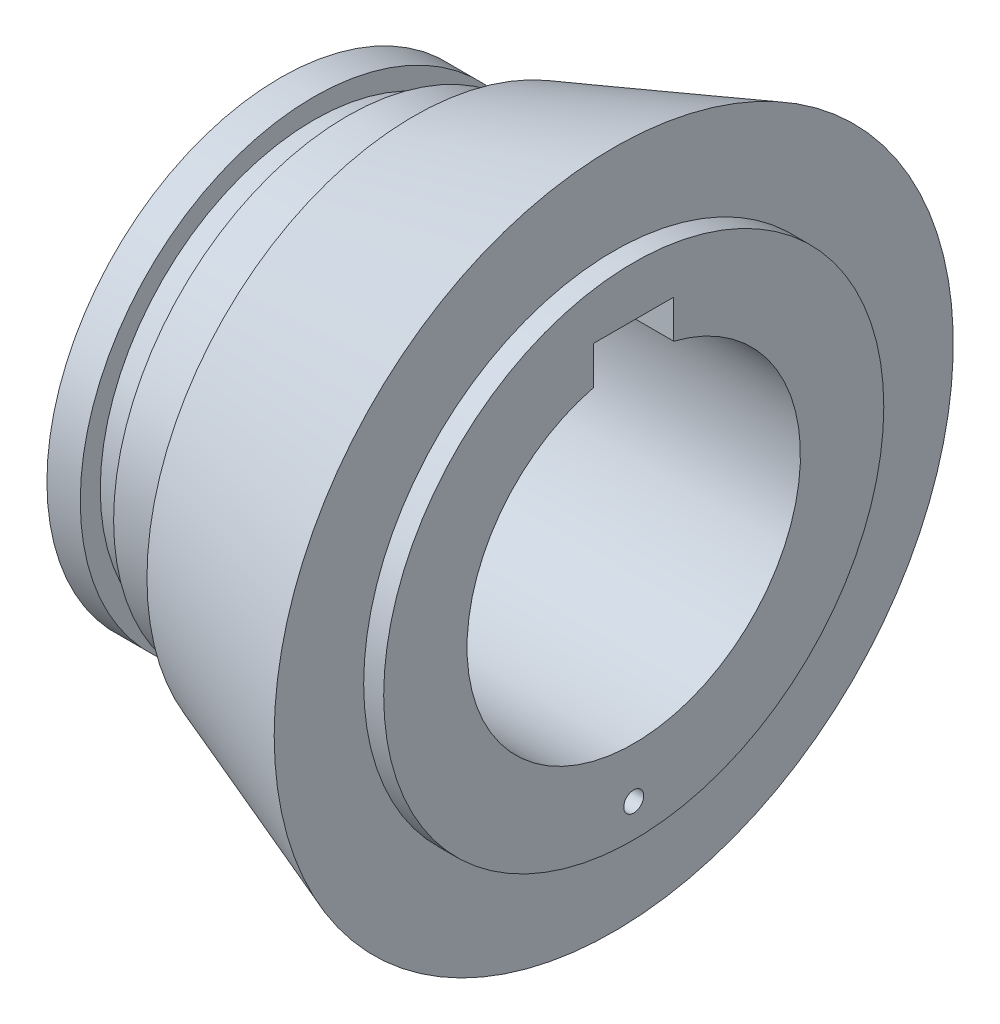
SolidWorks part; units mm, degrees
ref_plane "Front Plane" through (0, 0, 0) normal (0, 0, 1) x (1, 0, 0)
ref_plane "Top Plane" through (0, 0, 0) normal (0, 1, 0) x (1, 0, 0)
ref_plane "Right Plane" through (0, 0, 0) normal (1, 0, 0) x (0, 0, -1)
sketch "Sketch1" plane through (0, 0, 0) normal (0, 0, 1) x (1, 0, 0)
  line L0 (0, 0) -> (87.2965, 0) construction
  line L1 (0, 25) -> (0, 35)
  line L2 (0, 35) -> (5, 35)
  line L3 (5, 35) -> (5, 32)
  line L4 (5, 32) -> (10, 32)
  line L5 (10, 32) -> (10, 35)
  line L6 (10, 35) -> (20, 35)
  line L7 (20, 35) -> (20, 40)
  line L8 (20, 40) -> (50, 50.9191)
  line L9 (50, 50.9191) -> (50, 37.5)
  line L10 (50, 37.5) -> (53, 37.5)
  line L11 (53, 37.5) -> (53, 25)
  line L12 (53, 25) -> (0, 25)
  dimension "D1" = 53
  dimension "D2" = 3
  dimension "D3" = 25
  dimension "D4" = 35
  dimension "D5" = 37.5
  dimension "D6" = 40
  dimension "D7" = 5
  dimension "D8" = 5
  dimension "D9" = 3
  dimension "D10" = 35
  dimension "D11" = 10
  dimension "D12" = 20
revolve "Revolve1" add sketch "Sketch1" angle 360 about L0
sketch "Sketch2" plane through (53, 0, 0) normal (1, 0, 0) x (0, 0, -1)
  line L1 (-6, 30) -> (6, 30)
  line L2 (-6, 30) -> (-6, 18)
  line L3 (-6, 18) -> (6, 18)
  line L4 (6, 30) -> (6, 18)
  line L5 (-6, 30) -> (6, 18) construction
  line L6 (-6, 18) -> (6, 30) construction
  circle A0 centre (0, 0) radius 25 construction
  point P0 (0, 24)
  dimension "D2" = 30
  dimension "D1" = 12
  dimension "D3" = 0
extrude "Cut-Extrude1" cut sketch "Sketch2" against normal through all
sketch "Sketch3" plane through (53, 0, 0) normal (1, 0, 0) x (0, 0, -1)
  circle A0 centre (0, 0) radius 32.5 construction
  circle A1 centre (0, -32.5) radius 1.5
  dimension "D1" = 65
  dimension "D2" = 3
extrude "Cut-Extrude2" cut sketch "Sketch3" against normal blind 10
